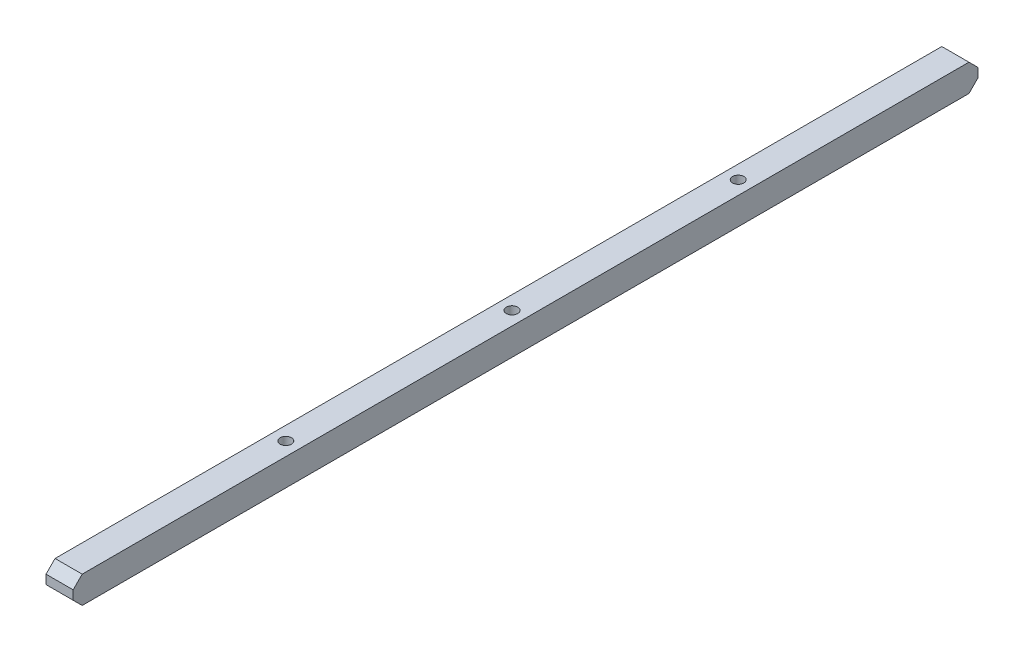
from build123d import *

# Parameters (mm, degrees)
SKETCH_1_W         = 6
SKETCH_1_H         = 6
EXTRUDE_1_DEPTH    = 200
HOLE_WIZARD_M3_1_D = 2.5
CHAMFER_1_SIZE     = 2


with BuildPart() as part:
    # 草图1 → 凸台-拉伸1 (new body)
    with BuildSketch(Plane.XY):
        Rectangle(SKETCH_1_W, SKETCH_1_H)
    extrude(amount=EXTRUDE_1_DEPTH)

    # M3 螺纹孔1 (through all)
    with Locations(Plane(origin=(0, 3, 50), x_dir=(0, 0, 1), z_dir=(0, 1, 0))):
        with Locations((0, 0), (50, 0), (100, 0)):
            Hole(HOLE_WIZARD_M3_1_D / 2)

    # 倒角1
    chamfer_1_edges = [part.edges().sort_by_distance(p)[0] for p in [
        (0, -3, 200),
        (0, -3, 0),
        (0, 3, 0),
        (0, 3, 200),
    ]]
    chamfer(chamfer_1_edges, length=CHAMFER_1_SIZE)


solid = part.part
